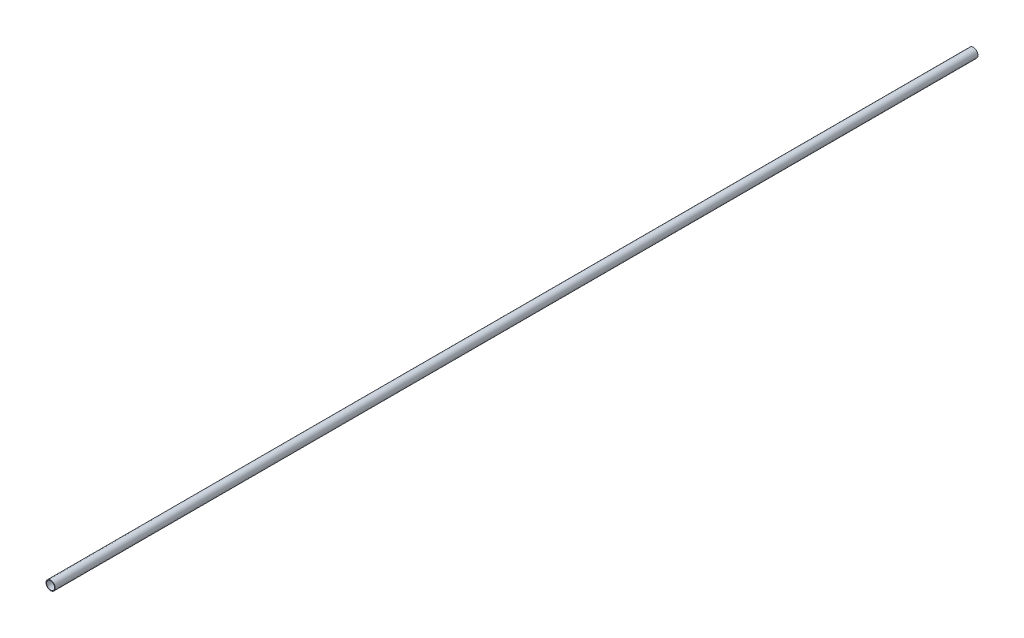
from build123d import *

# Parameters (mm, degrees)
SKETCH_1_R      = 16
SKETCH_1_R_2    = 14
EXTRUDE_1_DEPTH = 1600


with BuildPart() as part:
    # 草图1 → 凸台-拉伸1 (new, symmetric)
    with BuildSketch(Plane.XY):
        Circle(SKETCH_1_R)
        Circle(SKETCH_1_R_2, mode=Mode.SUBTRACT)
    extrude(amount=EXTRUDE_1_DEPTH, both=True)


solid = part.part
